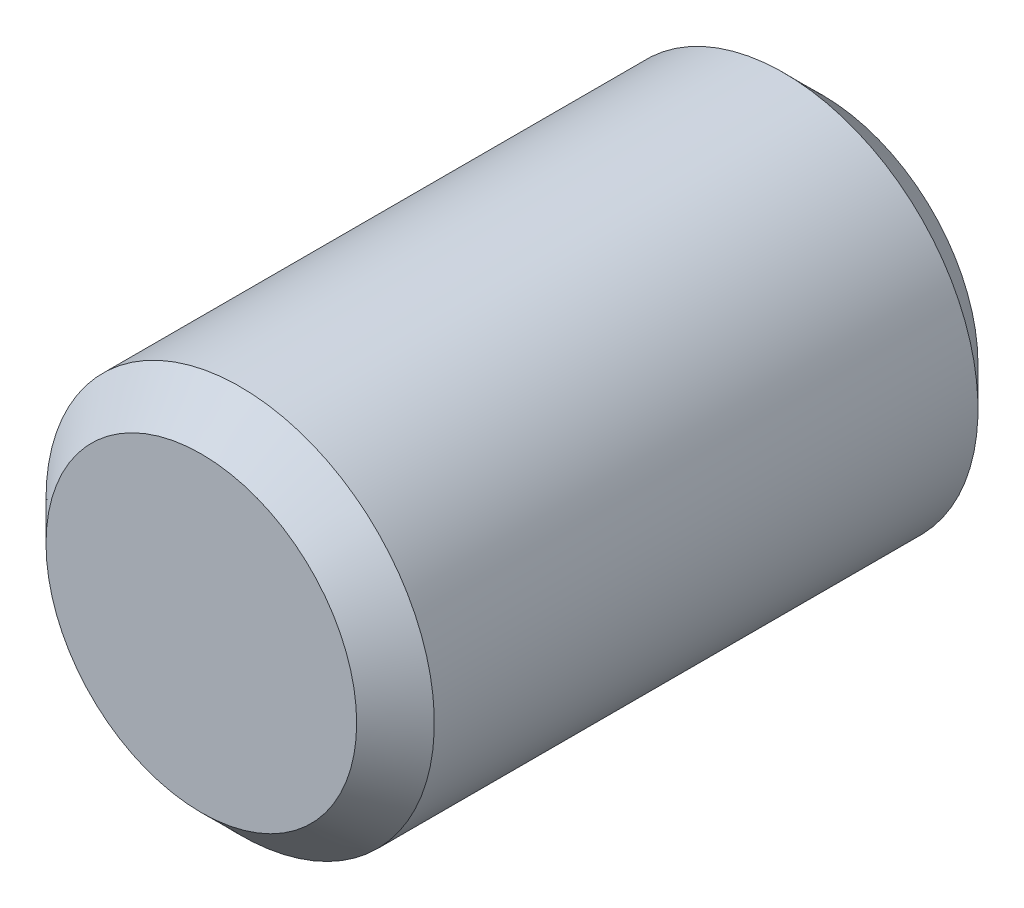
SolidWorks part; units mm, degrees
ref_plane "Front Plane" through (0, 0, 0) normal (0, 0, 1) x (1, 0, 0)
ref_plane "Top Plane" through (0, 0, 0) normal (0, 1, 0) x (1, 0, 0)
ref_plane "Right Plane" through (0, 0, 0) normal (1, 0, 0) x (0, 0, -1)
other "Configuration Table"
ref_plane "Plane1" through (0, 0, 0) normal (0, -1, 0) x (1, 0, 0)
sketch "Sketch1" plane through (0, 0, 0) normal (0, -1, 0) x (1, 0, 0)
  line L0 (2, 8) -> (0, 8)
  line L1 (0, 8) -> (0, 0)
  line L2 (0, 0) -> (2, 0)
  line L3 (2, 0) -> (2.5, 0.5)
  line L4 (2.5, 0.5) -> (2.5, 7.5)
  line L5 (2.5, 7.5) -> (2, 8)
  line L6 (0, 8) -> (0, 0) construction
revolve "Revolve1" add sketch "Sketch1" angle 360 about L6
